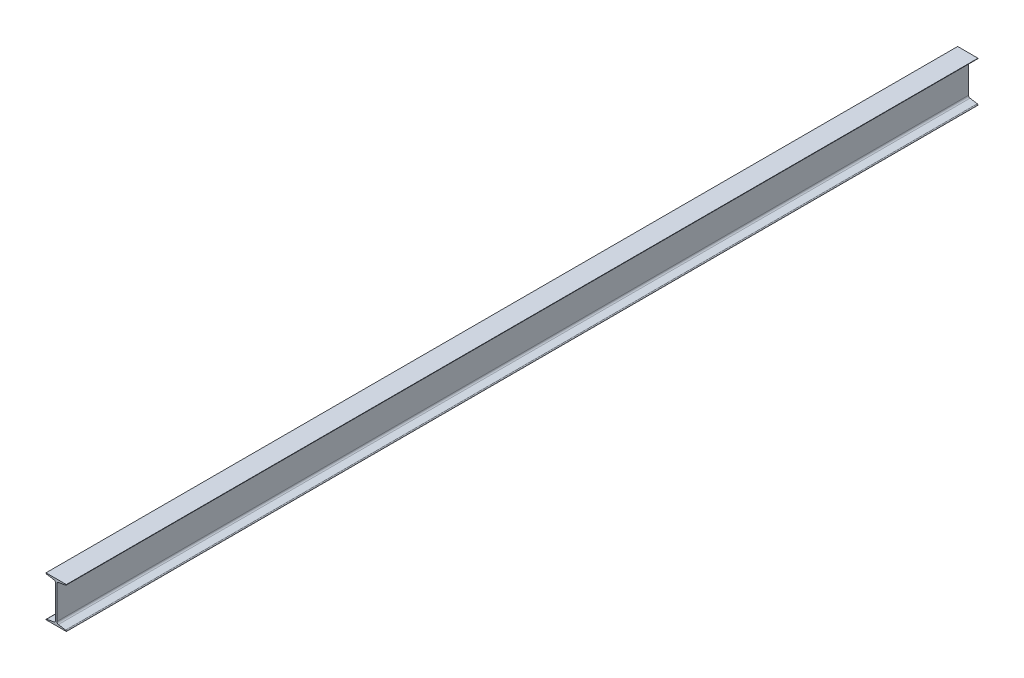
from build123d import *

# Parameters (mm, degrees)
BOSS_EXTRUDE1_DEPTH = 3580
MOVE_FACE1_BY       = 900


with BuildPart() as part:
    # Sketch1 → Boss-Extrude1 (new body)
    with BuildSketch(Plane.XY):
        with BuildLine():
            Line((314.404628659, 42.201600466), (314.404628659, -38.613650919))
            ThreePointArc((314.404628659, -38.613650919), (316.537566708, -44.431164147), (321.925397583, -47.491256194))
            Line((321.925397583, -47.491256194), (357.144244197, -53.359596897))
            ThreePointArc((357.144244197, -53.359596897), (359.838159635, -54.88964292), (360.904628659, -57.798399534))
            Line((360.904628659, -57.798399534), (310.904628659, -57.798399534))
            Line((310.904628659, -57.798399534), (260.904628659, -57.798399534))
            ThreePointArc((260.904628659, -57.798399534), (261.971097684, -54.88964292), (264.665013121, -53.359596897))
            Line((264.665013121, -53.359596897), (299.883859735, -47.491256194))
            ThreePointArc((299.883859735, -47.491256194), (305.27169061, -44.431164147), (307.404628659, -38.613650919))
            Line((307.404628659, -38.613650919), (307.404628659, 42.201600466))
            Line((307.404628659, 42.201600466), (307.404628659, 123.016851851))
            ThreePointArc((307.404628659, 123.016851851), (305.27169061, 128.834365079), (299.883859735, 131.894457126))
            Line((299.883859735, 131.894457126), (264.665013121, 137.762797828))
            ThreePointArc((264.665013121, 137.762797828), (261.971097684, 139.292843852), (260.904628659, 142.201600466))
            Line((260.904628659, 142.201600466), (310.904628659, 142.201600466))
            Line((310.904628659, 142.201600466), (360.904628659, 142.201600466))
            ThreePointArc((360.904628659, 142.201600466), (359.838159635, 139.292843852), (357.144244197, 137.762797828))
            Line((357.144244197, 137.762797828), (321.925397583, 131.894457126))
            ThreePointArc((321.925397583, 131.894457126), (316.537566708, 128.834365079), (314.404628659, 123.016851851))
            Line((314.404628659, 123.016851851), (314.404628659, 42.201600466))
        make_face()
    extrude(amount=BOSS_EXTRUDE1_DEPTH)

    # Move Face1: a face moved outward by 900.0
    extrude(part.faces().sort_by_distance((310.904628659, 42.201600466, 0))[0], amount=MOVE_FACE1_BY, dir=(0, 0, -1))


solid = part.part
